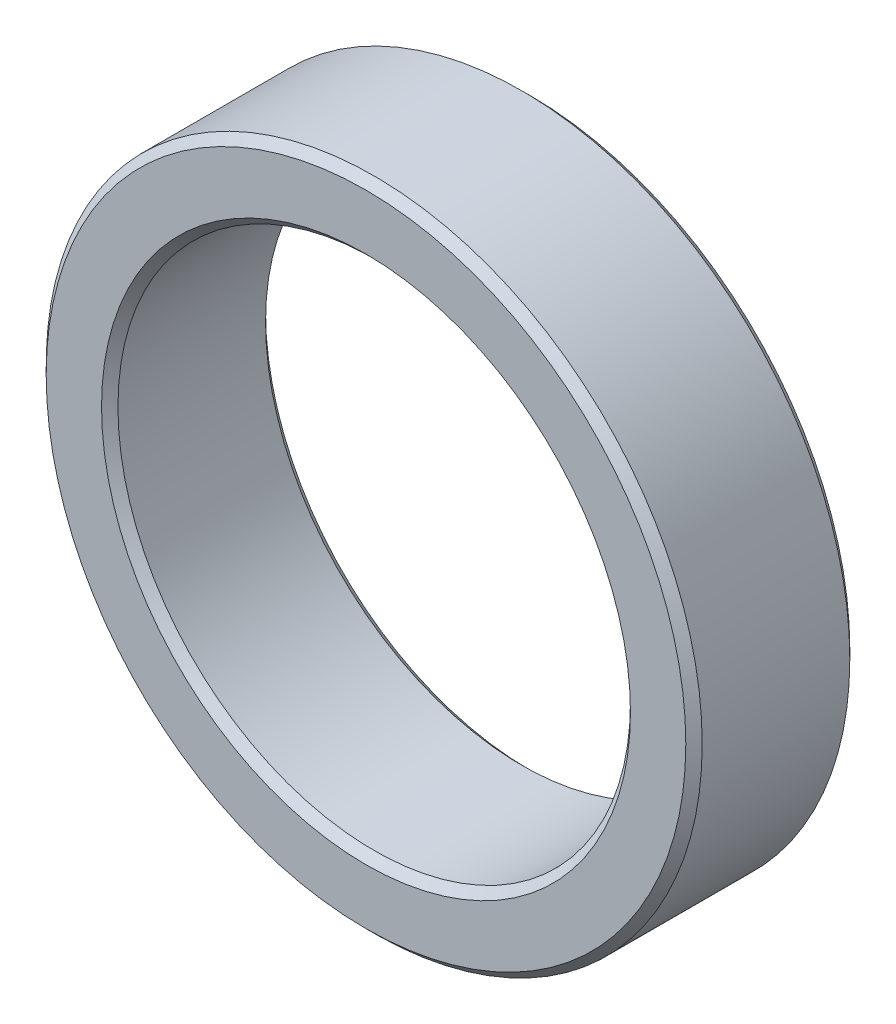
SolidWorks part; units mm, degrees
material "SUS304"
ref_plane "Front Plane" through (0, 0, 0) normal (0, 0, 1) x (1, 0, 0)
ref_plane "Top Plane" through (0, 0, 0) normal (0, 1, 0) x (1, 0, 0)
ref_plane "Right Plane" through (0, 0, 0) normal (1, 0, 0) x (0, 0, -1)
sketch "Sketch1" plane through (0, 0, 0) normal (0, 0, 1) x (1, 0, 0)
  circle A0 centre (0, 0) radius 8
  circle A1 centre (0, 0) radius 6.25
  dimension "D1" = 12.5
  dimension "D2" = 16
extrude "Boss-Extrude1" add sketch "Sketch1" along normal mid plane 4
chamfer "Chamfer1" distance 0.2 angle 45 4 edges at (6.25, 0, 2) (8, 0, 2) (6.25, 0, -2) (8, 0, -2)
